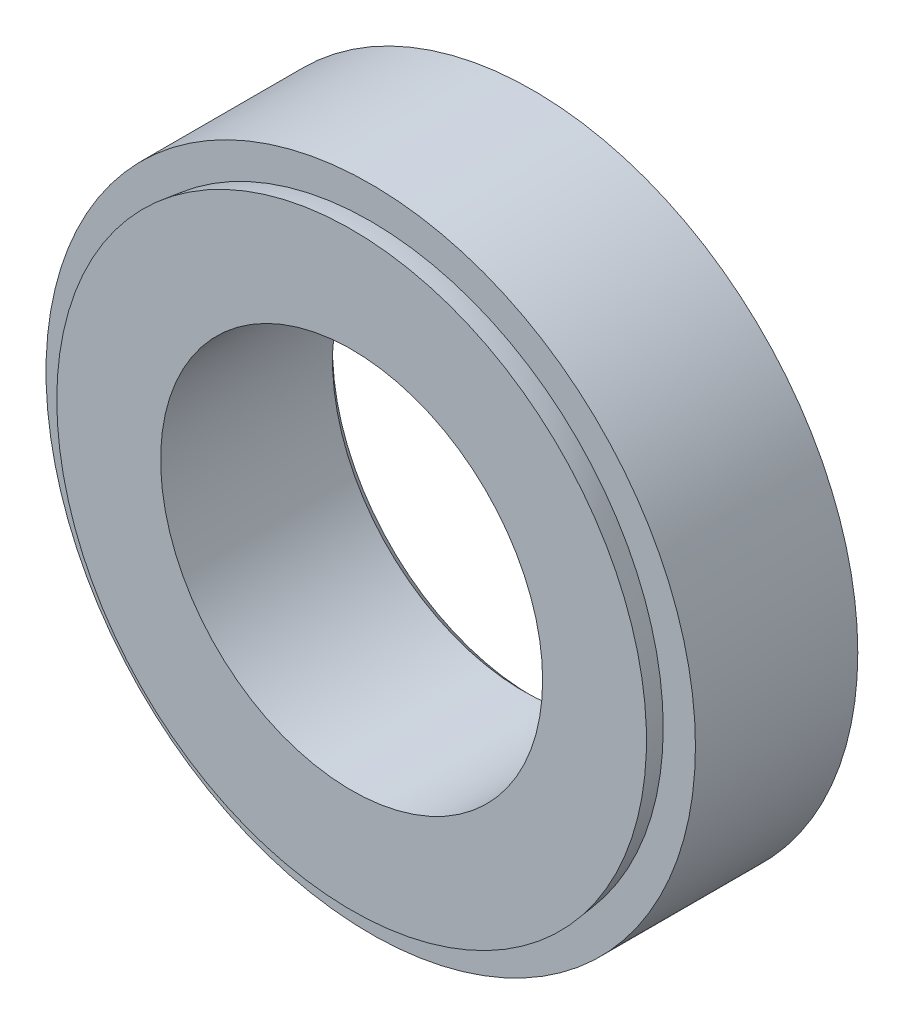
SolidWorks part; units mm, degrees
material "普通碳钢"
ref_plane "前视" through (0, 0, 0) normal (0, 0, 1) x (1, 0, 0)
ref_plane "上视" through (0, 0, 0) normal (0, 1, 0) x (1, 0, 0)
ref_plane "右视" through (0, 0, 0) normal (1, 0, 0) x (0, 0, -1)
sketch "草图1" plane through (0, 0, 0) normal (0, 0, 1) x (1, 0, 0)
  line L0 (0, 42.1384) -> (0, -37.7816) construction
  line L1 (-42.5891, 0) -> (41.1356, 0) construction
  circle A0 centre (0, 0) radius 34
  dimension "D1" = 68
extrude "凸台-拉伸1" add sketch "草图1" along normal blind 19 contours A0
sketch "草图2" plane through (0, 0, 0) normal (0, 1, 0) x (1, 0, 0)
  line L0 (-34, -19) -> (34, -19) construction
  line L1 (-34, -17) -> (-30.6261, -17)
  line L2 (-30.8733, -19) -> (-34, -19)
  line L3 (-34, -19) -> (-34, -17)
  arc A0 (-30.6261, -17) -> (-30.8733, -19) centre (0, -21.8) ccw
  dimension "D1" = 2.8
  dimension "D2" = 62
  dimension "D4" = 2
revolve "切除-旋转1" cut sketch "草图2" angle 360 about axis through (0, 0, 19) along (0, 0, -1)
sketch "草图3" plane through (0, 0, 19) normal (0, 0, 1) x (1, 0, 0)
  circle A0 centre (0, 0) radius 20
  dimension "D1" = 40
extrude "切除-拉伸1" cut sketch "草图3" against normal through all
chamfer "倒角1" distance 1 angle 45 1 edges at (20, 0, 0)
